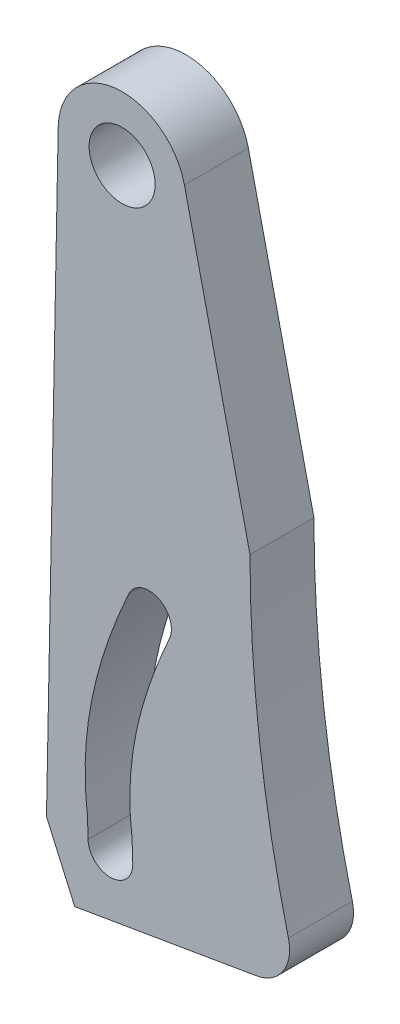
from build123d import *

# Parameters (mm, degrees)
SKETCH_1_R      = 1.55
EXTRUDE_1_DEPTH = 3


with BuildPart() as part:
    # 草图1 (on Front Plane) → 凸台-拉伸1 (new body)
    with BuildSketch(Plane.XY):
        with BuildLine():
            Line((3.816218697, 0.711369777), (0.741076539, 14.191366792))
            ThreePointArc((0.741076539, 14.191366792), (-2.49053861, 16.508405149), (-5.183215516, 13.582402021))
            Line((-5.183215516, 13.582402021), (-5.732788153, -14.705577537))
            Line((-5.732788153, -14.705577537), (-4.408096335, -17.704776028))
            Line((-4.408096335, -17.704776028), (4.127837654, -16.252589359))
            ThreePointArc((4.127837654, -16.252589359), (5.371423242, -15.437528643), (5.619036958, -13.971405684))
            ThreePointArc((5.619036958, -13.971405684), (4.268609288, -6.685150501), (3.816218697, 0.711369777))
        make_face()
        with Locations((-2.183781514, 13.524129678)):
            Circle(SKETCH_1_R, mode=Mode.SUBTRACT)
        with BuildLine():
            ThreePointArc((-3.783386383, -14.657279108), (-2.707701661, -15.680950138), (-1.684030631, -14.605265415))
            add(Edge.make_bspline(
                [(-1.684030631, -14.605265415), (-1.698385943, -14.230913496), (-1.690645088, -13.65109076), (-1.790811076, -12.90815818), (-1.819576713, -12.363575922), (-1.822848669, -11.844967012), (-1.807105928, -11.320378821), (-1.768151471, -10.788389789), (-1.707646295, -10.25185083), (-1.625402268, -9.709964922), (-1.486001031, -8.974109842), (-1.351215721, -8.423808693), (-1.249236023, -8.057041386)],
                knots=[0, 0, 0, 0, 0.170354994, 0.26229743, 0.340043602, 0.417823563, 0.497759338, 0.578301179, 0.659976625, 0.742887413, 0.827131807, 1, 1, 1, 1], degree=3))
            add(Edge.make_bspline(
                [(0.03013882, -4.613074169), (-0.143309735, -4.996054164), (-0.391510935, -5.572837816), (-0.692509933, -6.347460357), (-0.964714861, -7.105557392), (-1.143447826, -7.676581339), (-1.249236023, -8.057041386)],
                knots=[0, 0, 0, 0, 0.342979707, 0.512099324, 0.677879853, 1, 1, 1, 1], degree=3))
            ThreePointArc((0.03013882, -4.613074169), (-0.488256217, -3.213540285), (-1.882444762, -3.746144084))
            add(Edge.make_bspline(
                [(-3.783386383, -14.657279108), (-3.799290999, -14.2981548), (-3.786309002, -13.774144994), (-3.886484574, -13.055813522), (-3.915903208, -12.486133418), (-3.923833984, -11.87345296), (-3.906620769, -11.257653943), (-3.849073975, -10.432184554), (-3.741043656, -9.603680421), (-3.586380227, -8.77634916), (-3.446679883, -8.151733856), (-3.28447898, -7.525898679), (-3.10051603, -6.898880381), (-2.895571139, -6.270661953), (-2.670469593, -5.64113868), (-2.342560405, -4.794442901), (-2.072047563, -4.164799113), (-1.882444762, -3.746144084)],
                knots=[0, 0, 0, 0, 0.096210271, 0.139297547, 0.1935541, 0.248477319, 0.302979464, 0.358078206, 0.469497102, 0.525932365, 0.582904263, 0.640455034, 0.69862477, 0.757451361, 0.816970378, 0.877214945, 1, 1, 1, 1], degree=3))
        make_face(mode=Mode.SUBTRACT)
    extrude(amount=EXTRUDE_1_DEPTH)


solid = part.part
